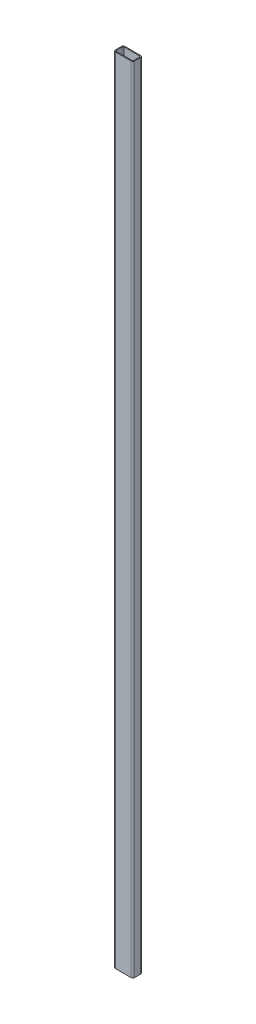
SolidWorks part; units mm, degrees
ref_plane "Front" through (0, 0, 0) normal (0, 0, 1) x (1, 0, 0)
ref_plane "Top" through (0, 0, 0) normal (0, 1, 0) x (1, 0, 0)
ref_plane "Right" through (0, 0, 0) normal (1, 0, 0) x (0, 0, -1)
sketch "草图1" plane through (0, 0, 0) normal (0, 1, 0) x (1, 0, 0)
  line L0 (-16, -8) -> (16, -8)
  line L1 (-16, -10) -> (16, -10)
  line L2 (-20, -6) -> (-20, 6)
  line L3 (-16, 10) -> (16, 10)
  line L4 (20, -6) -> (20, 6)
  line L5 (-20, -10) -> (20, 10) construction
  line L6 (-20, 10) -> (20, -10) construction
  line L7 (18, -6) -> (18, 6)
  line L8 (-16, 8) -> (16, 8)
  line L9 (-18, -6) -> (-18, 6)
  arc A0 (-16, -10) -> (-20, -6) centre (-16, -6) cw
  arc A1 (16, -10) -> (20, -6) centre (16, -6) ccw
  arc A2 (16, 10) -> (20, 6) centre (16, 6) cw
  arc A3 (-20, 6) -> (-16, 10) centre (-16, 6) cw
  arc A4 (16, -8) -> (18, -6) centre (16, -6) ccw
  arc A5 (16, 8) -> (18, 6) centre (16, 6) cw
  arc A6 (-18, 6) -> (-16, 8) centre (-16, 6) cw
  arc A7 (-16, -8) -> (-18, -6) centre (-16, -6) cw
  point P0 (0, 0)
  dimension "D3" = 4
  dimension "D1" = 40
  dimension "D2" = 20
  dimension "D4" = 2
extrude "凸台-拉伸1" add sketch "草图1" along normal blind 1650
